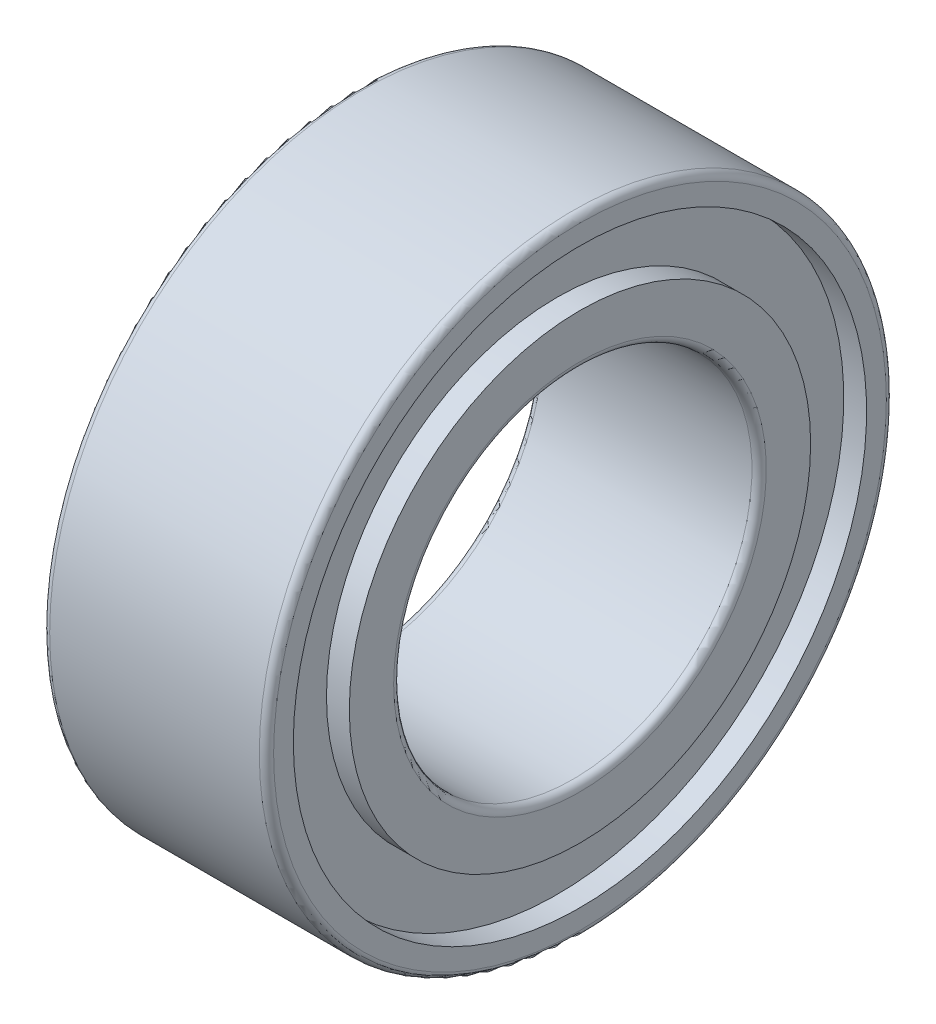
from build123d import *


with BuildPart() as part:
    # Sketch1 → Revolve1 (revolve)
    with BuildSketch(Plane.XY, mode=Mode.PRIVATE) as revolve1_sk:
        with BuildLine():
            Line((0, 3.42), (0, 3.2))
            Line((0, 3.2), (0.255, 3.2))
            Line((0.255, 3.2), (0.255, 2.575))
            Line((0.255, 2.575), (0, 2.575))
            Line((0, 2.575), (0, 2.08))
            ThreePointArc((0, 2.08), (0.023431458, 2.023431458), (0.08, 2))
            Line((0.08, 2), (2.42, 2))
            ThreePointArc((2.42, 2), (2.476568542, 2.023431458), (2.5, 2.08))
            Line((2.5, 2.08), (2.5, 2.575))
            Line((2.5, 2.575), (2.245, 2.575))
            Line((2.245, 2.575), (2.245, 3.2))
            Line((2.245, 3.2), (2.5, 3.2))
            Line((2.5, 3.2), (2.5, 3.42))
            ThreePointArc((2.5, 3.42), (2.476568542, 3.476568542), (2.42, 3.5))
            Line((2.42, 3.5), (0.08, 3.5))
            ThreePointArc((0.08, 3.5), (0.023431458, 3.476568542), (0, 3.42))
        make_face()
    revolve(revolve1_sk.sketch.rotate(Axis((2.42, 0, 0), (-1, 0, 0)), 270), axis=Axis((2.42, 0, 0), (-1, 0, 0)))


solid = part.part
